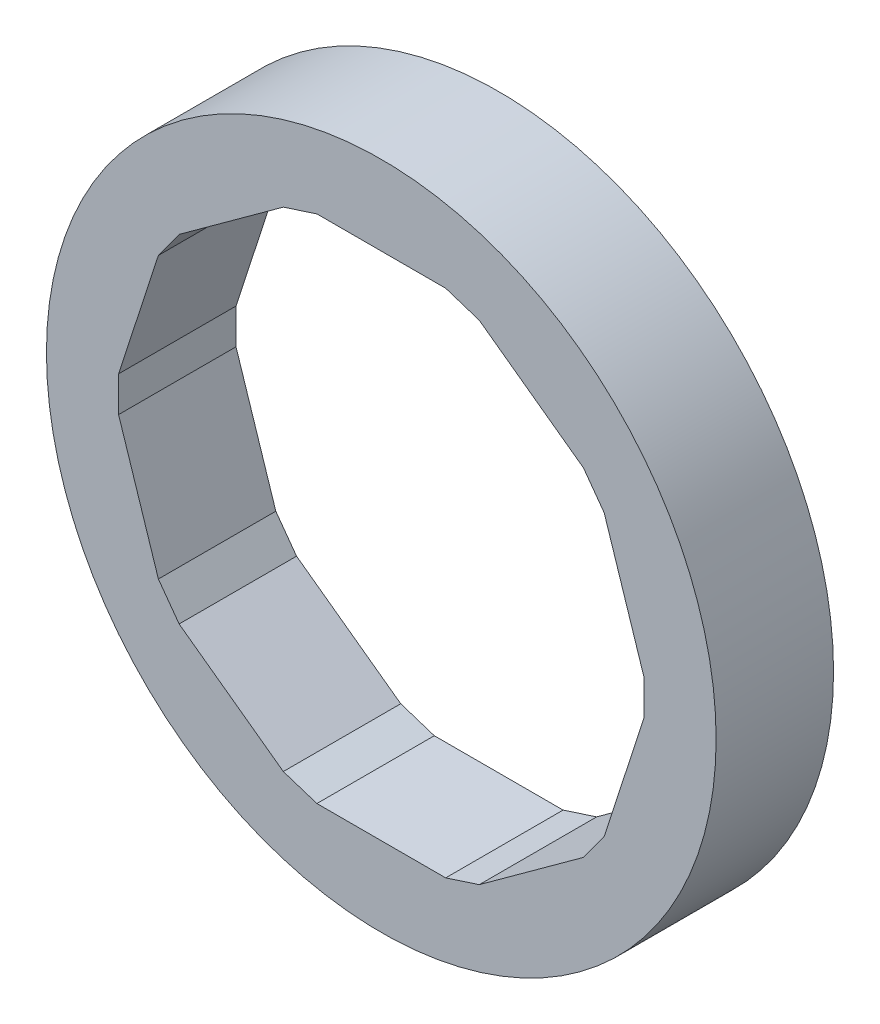
SolidWorks part; units mm, degrees
ref_plane "前视基准面" through (0, 0, 0) normal (0, 0, 1) x (1, 0, 0)
ref_plane "上视基准面" through (0, 0, 0) normal (0, 1, 0) x (1, 0, 0)
ref_plane "右视基准面" through (0, 0, 0) normal (1, 0, 0) x (0, 0, -1)
other "Configuration Table"
sketch "草图1" plane through (0, 0, 0) normal (0, 0, 1) x (1, 0, 0)
  line L20 (346.7725, -23.2989) -> (346.7725, 23.2989)
  line L21 (346.7725, -23.2989) -> (294.2396, -184.9785)
  line L22 (294.2396, -184.9785) -> (266.8501, -222.677)
  line L23 (266.8501, -222.677) -> (129.3172, -322.6005)
  line L24 (85, -337) -> (129.3172, -322.6005)
  line L25 (85, -337) -> (-85, -337)
  line L26 (-129.3172, -322.6005) -> (-85, -337)
  line L27 (-129.3172, -322.6005) -> (-266.8501, -222.677)
  line L28 (-294.2396, -184.9785) -> (-266.8501, -222.677)
  line L29 (-294.2396, -184.9785) -> (-346.7725, -23.2989)
  line L30 (-346.7725, 23.2989) -> (-346.7725, -23.2989)
  line L31 (-346.7725, 23.2989) -> (-294.2396, 184.9785)
  line L32 (-266.8501, 222.677) -> (-294.2396, 184.9785)
  line L33 (-266.8501, 222.677) -> (-129.3172, 322.6005)
  line L34 (-85, 337) -> (85, 337)
  line L35 (-85, 337) -> (-129.3172, 322.6005)
  line L36 (129.3172, 322.6005) -> (85, 337)
  line L37 (129.3172, 322.6005) -> (266.8501, 222.677)
  line L38 (294.2396, 184.9785) -> (266.8501, 222.677)
  line L39 (294.2396, 184.9785) -> (346.7725, 23.2989)
  circle A0 centre (0, 0) radius 442
  dimension "D1" = 884
extrude "凸台-拉伸1" add sketch "草图1" along normal mid plane 155
